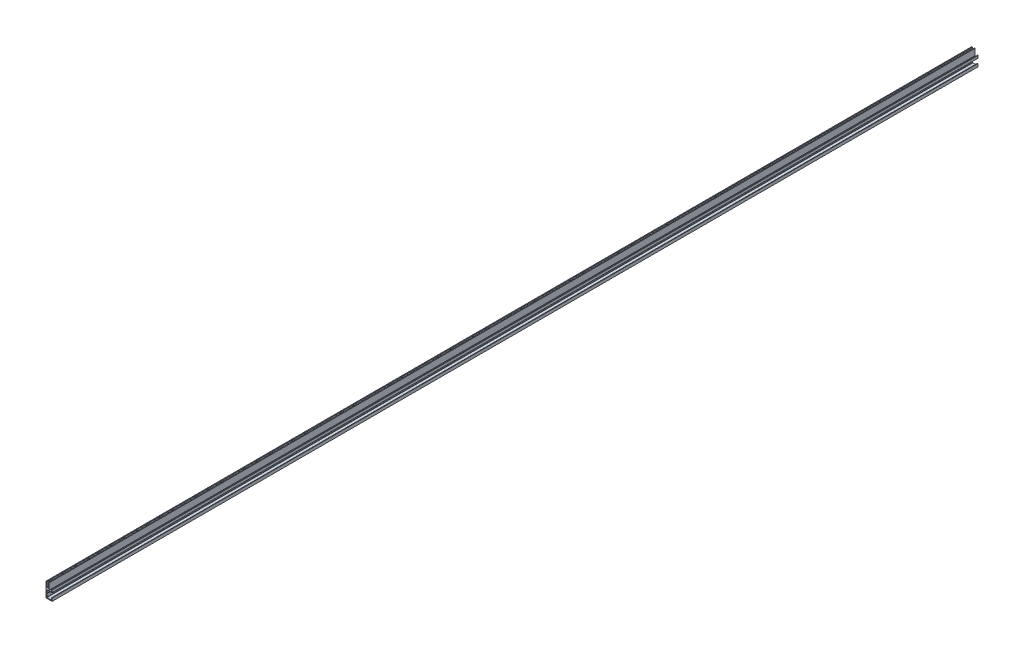
from build123d import *

# Parameters (mm, degrees)
EXTRUDE_1_DEPTH = 1108


with BuildPart() as part:
    # 草图2 → 凸台-拉伸1 (new, symmetric)
    with BuildSketch(Plane.XY):
        with BuildLine():
            Line((14.484958611, 7.149447031), (13.704975481, 7.149447031))
            ThreePointArc((13.704975481, 7.149447031), (13.280736974, 6.973721688), (13.105011631, 6.549483181))
            Line((13.105011631, 6.549483181), (13.105011631, 2.269839045))
            ThreePointArc((13.105011631, 2.269839045), (13.06986594, 2.184990722), (12.985017102, 2.149846275))
            Line((12.985017102, 2.149846275), (2.5, 2.15))
            ThreePointArc((2.5, 2.15), (2.146446609, 2.296446609), (2, 2.65))
            Line((2, 2.65), (2, 9.75))
            ThreePointArc((2, 9.75), (1.75, 10), (2, 10.25))
            Line((2, 10.25), (2, 17.35))
            ThreePointArc((2, 17.35), (2.146446609, 17.703553391), (2.5, 17.85))
            Line((2.5, 17.85), (14.604187277, 17.85))
            Line((14.604187277, 17.85), (14.604187277, 23.829737701))
            ThreePointArc((14.604187277, 23.829737701), (14.569042208, 23.914585402), (14.484194507, 23.949730471))
            Line((14.484194507, 23.949730471), (13.704211377, 23.949730471))
            ThreePointArc((13.704211377, 23.949730471), (13.27997287, 23.774005128), (13.104247527, 23.349766621))
            Line((13.104247527, 23.349766621), (13.104247527, 19.46999277))
            ThreePointArc((13.104247527, 19.46999277), (13.069102458, 19.385145069), (12.984254757, 19.35))
            Line((12.984254757, 19.35), (7.2, 19.35))
            Line((7.2, 19.35), (7.2, 34.798393128))
            Line((7.2, 34.798393128), (6, 34.798393128))
            ThreePointArc((6, 34.798393128), (5.858578644, 34.739814485), (5.8, 34.598393128))
            Line((5.8, 34.598393128), (5.8, 33.098393128))
            ThreePointArc((5.8, 33.098393128), (5.7, 32.998393128), (5.8, 32.898393128))
            Line((5.8, 32.898393128), (5.8, 23.812239282))
            ThreePointArc((5.8, 23.812239282), (5.507106781, 23.105132501), (4.8, 22.812239282))
            Line((4.8, 22.812239282), (2.8, 22.812239282))
            ThreePointArc((2.8, 22.812239282), (2.092893219, 23.105132501), (1.8, 23.812239282))
            Line((1.8, 23.812239282), (1.8, 32.898393128))
            ThreePointArc((1.8, 32.898393128), (1.9, 32.998393128), (1.8, 33.098393128))
            Line((1.8, 33.098393128), (1.8, 34.598393128))
            ThreePointArc((1.8, 34.598393128), (1.741421356, 34.739814485), (1.6, 34.798393128))
            Line((1.6, 34.798393128), (0, 34.798393128))
            Line((0, 34.798393128), (0, 0))
            Line((0, 0), (14.6, 0))
            Line((14.6, 0), (14.604951381, 7.029454261))
            ThreePointArc((14.604951381, 7.029454261), (14.569806312, 7.114301962), (14.484958611, 7.149447031))
        make_face()
    extrude(amount=EXTRUDE_1_DEPTH, both=True)


solid = part.part
